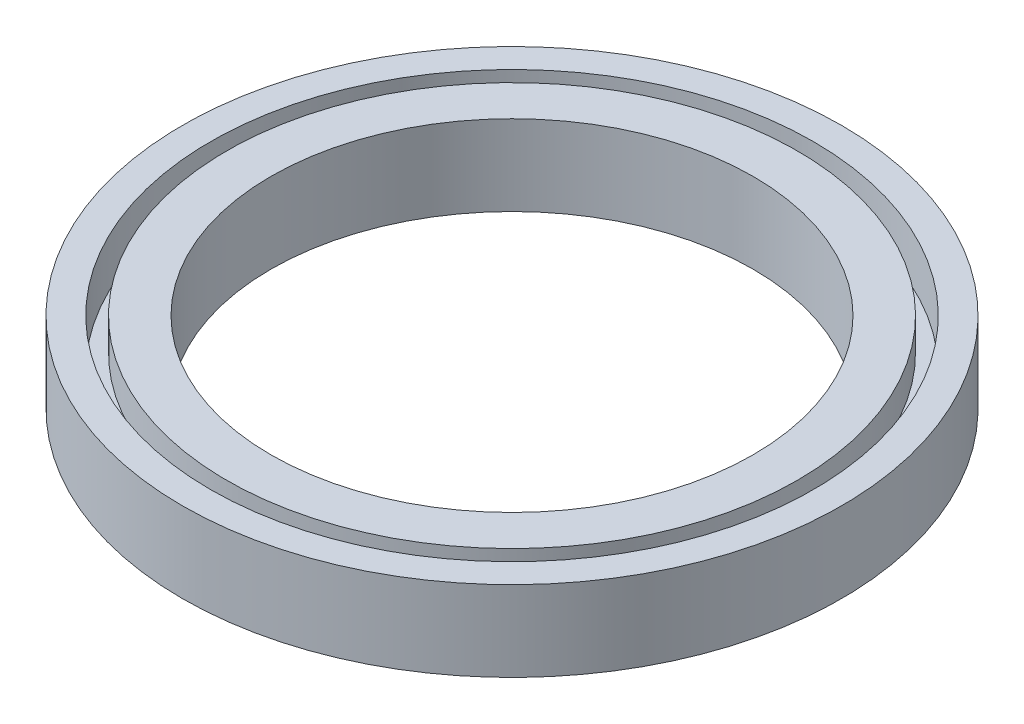
from build123d import *

# Parameters (mm, degrees)
SKETCH_1_R        = 16.25
SKETCH_1_R_2      = 15
EXTRUDE_1_DEPTH   = 5
SKETCH_1_R_3      = 20.5
SKETCH_1_R_4      = 18.75
EXTRUDE_1_2_DEPTH = 5
EXTRUDE_START     = -2
SKETCH_2_R        = 17.75
SKETCH_2_R_2      = 16.25
EXTRUDE_1_3_DEPTH = 2
SKETCH_3_R        = 18.75
SKETCH_3_R_2      = 17.25
EXTRUDE_2_DEPTH   = 2


with BuildPart() as part:
    # 草图1 → Extrude 1 (new body)
    with BuildSketch(Plane(origin=(0, 0, 0), x_dir=(1, 0, 0), z_dir=(0, 1, 0))):
        with Locations(Location((0, 0, 0), (0, 0, 270))):
            Circle(SKETCH_1_R)
        with Locations(Location((0, 0, 0), (0, 0, 270))):
            Circle(SKETCH_1_R_2, mode=Mode.SUBTRACT)
    extrude(amount=EXTRUDE_1_DEPTH)

    # 草图2 → Extrude 1 3 (add)
    with BuildSketch(Plane(origin=(0, 5, 0), x_dir=(1, 0, 0), z_dir=(0, 1, 0)).offset(EXTRUDE_START)):
        Circle(SKETCH_2_R)
        Circle(SKETCH_2_R_2, mode=Mode.SUBTRACT)
    extrude(amount=EXTRUDE_1_3_DEPTH)


with BuildPart() as body_2:
    # 草图1 → Extrude 1 2 (new body)
    with BuildSketch(Plane(origin=(0, 0, 0), x_dir=(1, 0, 0), z_dir=(0, 1, 0))):
        with Locations(Location((0, 0, 0), (0, 0, 270))):
            Circle(SKETCH_1_R_3)
        with Locations(Location((0, 0, 0), (0, 0, 270))):
            Circle(SKETCH_1_R_4, mode=Mode.SUBTRACT)
    extrude(amount=EXTRUDE_1_2_DEPTH)

    # 草图3 → 拉伸-薄壁2 (add)
    with BuildSketch(Plane.XZ):
        Circle(SKETCH_3_R)
        Circle(SKETCH_3_R_2, mode=Mode.SUBTRACT)
    extrude(amount=-EXTRUDE_2_DEPTH)


solid = Compound([part.part, body_2.part])
